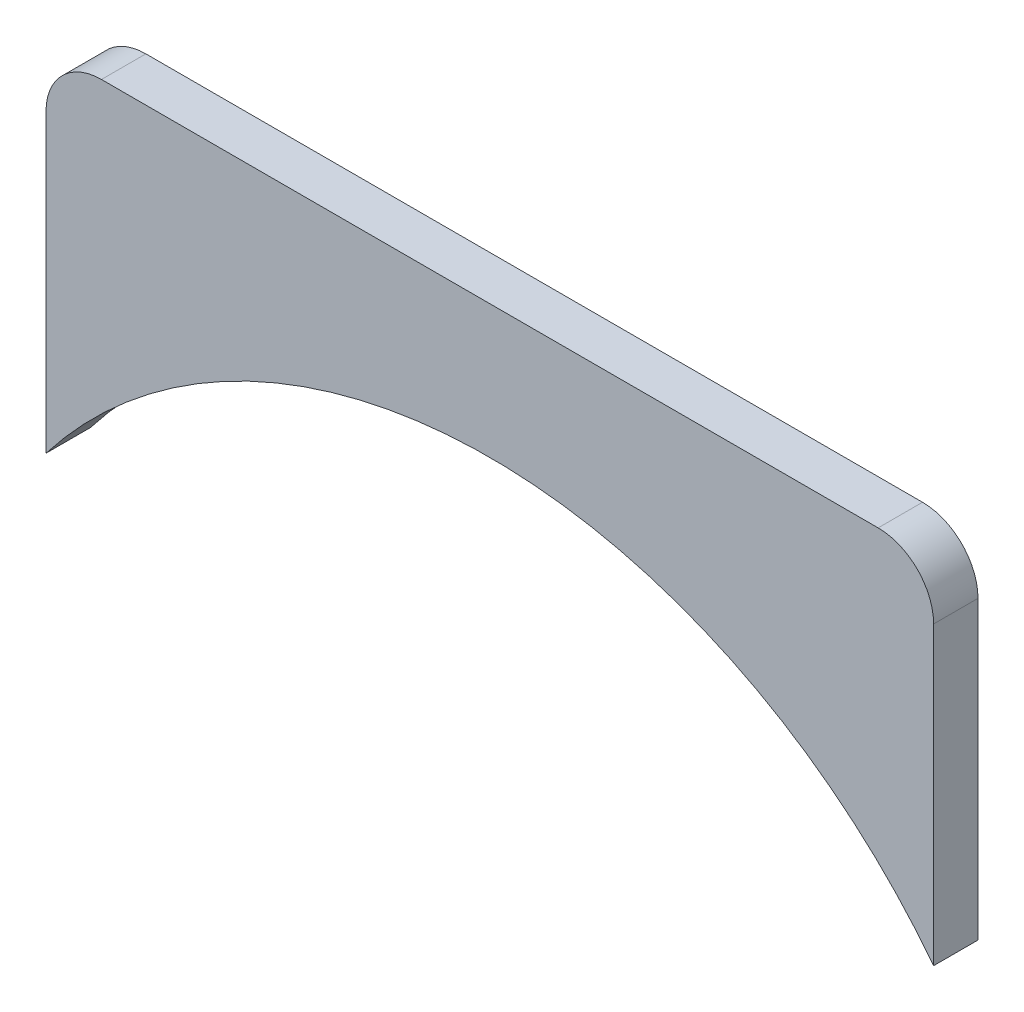
SolidWorks part; units mm, degrees
material "Q235B"
ref_plane "Front Plane" through (0, 0, 0) normal (0, 0, 1) x (1, 0, 0)
ref_plane "Top Plane" through (0, 0, 0) normal (0, 1, 0) x (1, 0, 0)
ref_plane "Right Plane" through (0, 0, 0) normal (1, 0, 0) x (0, 0, -1)
sketch "Sketch1" plane through (0, 0, 0) normal (0, 0, 1) x (1, 0, 0)
  line L0 (0, 0) -> (0, 64.4176) construction
  line L1 (80, 125) -> (-80, 125)
  line L2 (-80, 125) -> (-80, 61.6523)
  line L3 (80, 125) -> (80, 61.6523)
  arc A1 (80, 61.6523) -> (-80, 61.6523) centre (0, 0) ccw
  dimension "D1" = 101
  dimension "D2" = 125
  dimension "D3" = 160
extrude "Boss-Extrude1" add sketch "Sketch1" along normal blind 8
fillet "Fillet1" radius 10 2 edges at (-80, 125, 4) (80, 125, 4)
